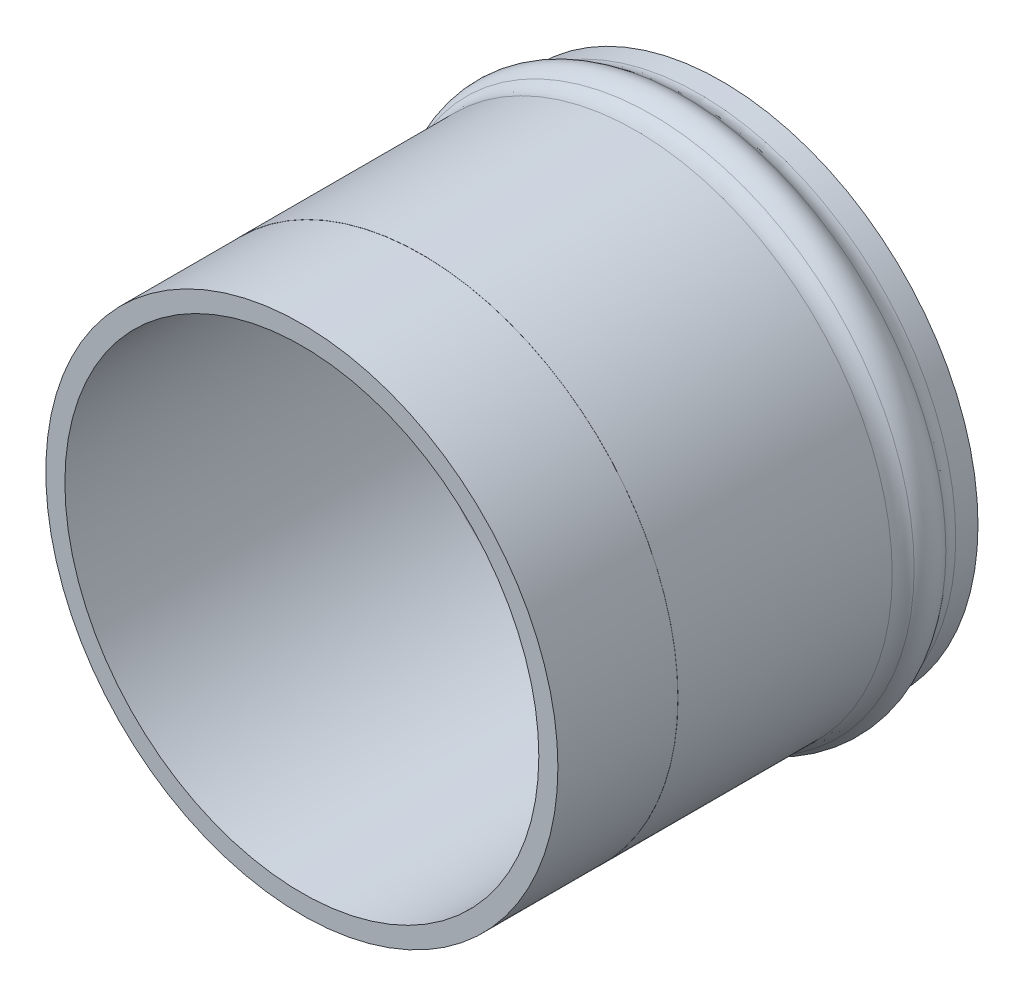
from build123d import *

# Parameters (mm, degrees)
CUT_EXTRUDE1_START = -10
SKETCH2_R          = 21.35
SKETCH2_R_2        = 21.34
CUT_EXTRUDE1_DEPTH = 10


with BuildPart() as part:
    # Sketch1 → Revolve-Thin1 (revolve)
    with BuildSketch(Plane(origin=(0, 0, 0), x_dir=(0, 0, -1), z_dir=(1, 0, 0)), mode=Mode.PRIVATE) as revolve_thin1_sk:
        with BuildLine():
            Line((0, 21.35), (27.854248689, 21.35))
            ThreePointArc((27.854248689, 21.35), (28.56135547, 21.479171307), (29.177124344, 21.85))
            ThreePointArc((29.177124344, 21.85), (30.5, 22.35), (31.822875656, 21.85))
            ThreePointArc((31.822875656, 21.85), (32.43864453, 21.479171307), (33.145751311, 21.35))
            Line((33.145751311, 21.35), (35, 21.35))
            Line((35, 21.35), (35, 19.75))
            Line((35, 19.75), (33.145751311, 19.75))
            ThreePointArc((33.145751311, 19.75), (31.872959105, 19.982508352), (30.764575131, 20.65))
            ThreePointArc((30.764575131, 20.65), (30.5, 20.75), (30.235424869, 20.65))
            ThreePointArc((30.235424869, 20.65), (29.127040895, 19.982508352), (27.854248689, 19.75))
            Line((27.854248689, 19.75), (0, 19.75))
            Line((0, 19.75), (0, 21.35))
        make_face()
    revolve(revolve_thin1_sk.sketch.rotate(Axis((0, 0, 0), (0, 0, -1)), 90), axis=Axis((0, 0, 0), (0, 0, -1)))

    # Sketch2 → Cut-Extrude1 (cut)
    with BuildSketch(Plane.XY.offset(CUT_EXTRUDE1_START)):
        Circle(SKETCH2_R)
        Circle(SKETCH2_R_2, mode=Mode.SUBTRACT)
    extrude(amount=CUT_EXTRUDE1_DEPTH, mode=Mode.SUBTRACT)


solid = part.part
